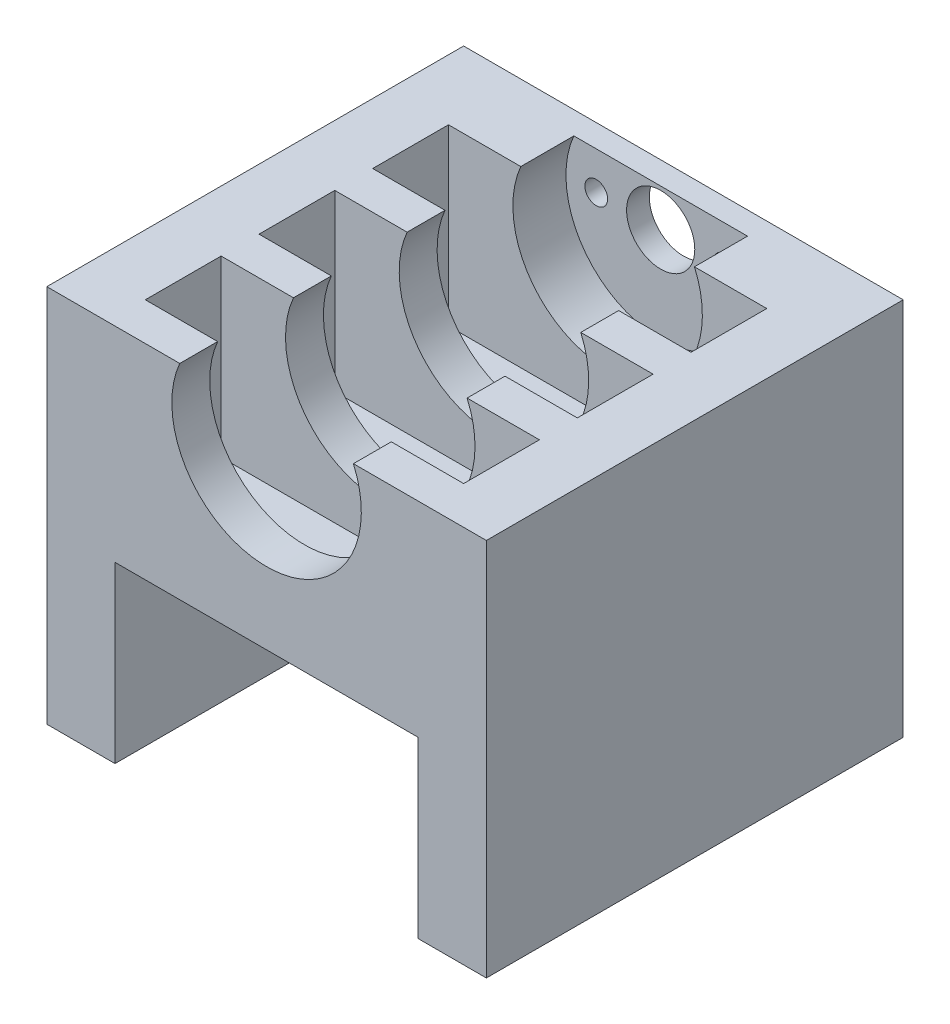
from build123d import *

# Parameters (mm, degrees)
SKETCH1_W             = 58
SKETCH1_H             = 50
BOSS_EXTRUDE1_DEPTH   = 55
SKETCH3_R             = 4.5
SKETCH3_R_2           = 1.5
CUT_EXTRUDE2_DEPTH    = 5
SKETCH2_R             = 12.5
CUT_EXTRUDE1_DEPTH    = 52
SKETCH4_W             = 40
SKETCH4_H             = 46
CUT_EXTRUDE3_DEPTH    = 70
M4_TAPPED_HOLE1_D     = 3.3
M4_TAPPED_HOLE1_DEPTH = 10.1
M4_TAPPED_HOLE1_TIP   = 0.991420021
SKETCH8_W             = 42
SKETCH8_H             = 10
CUT_EXTRUDE4_DEPTH    = 23


with BuildPart() as part:
    # Sketch1 → Boss-Extrude1 (new body)
    with BuildSketch(Plane.XY):
        Rectangle(SKETCH1_W, SKETCH1_H)
    extrude(amount=BOSS_EXTRUDE1_DEPTH)

    # Sketch3 → Cut-Extrude2 (cut)
    with BuildSketch(Plane(origin=(0, 0, 0), x_dir=(-1, 0, 0), z_dir=(0, 0, -1))):
        with Locations((0, 20)):
            Circle(SKETCH3_R)
        with Locations((-8.5, 20)):
            Circle(SKETCH3_R_2)
        with Locations((8.5, 20)):
            Circle(SKETCH3_R_2)
    extrude(amount=-CUT_EXTRUDE2_DEPTH, mode=Mode.SUBTRACT)

    # Sketch2 → Cut-Extrude1 (cut)
    with BuildSketch(Plane.XY.offset(55)):
        with Locations((0, 20)):
            Circle(SKETCH2_R)
    extrude(amount=-CUT_EXTRUDE1_DEPTH, mode=Mode.SUBTRACT)

    # Sketch4 → Cut-Extrude3 (cut)
    with BuildSketch(Plane(origin=(0, 0, 0), x_dir=(-1, 0, 0), z_dir=(0, 0, -1))):
        with Locations((0, -25)):
            Rectangle(SKETCH4_W, SKETCH4_H)
    extrude(amount=-CUT_EXTRUDE3_DEPTH, mode=Mode.SUBTRACT)

    # M4 Tapped Hole1
    with Locations(Plane(origin=(0, -25, 0), x_dir=(-1, 0, 0), z_dir=(0, -1, 0))):
        with Locations((24.5, -47), (24.5, -8), (-24.5, -8), (-24.5, -47)):
            Hole(M4_TAPPED_HOLE1_D / 2, depth=M4_TAPPED_HOLE1_DEPTH)
            with Locations((0, 0, -(M4_TAPPED_HOLE1_DEPTH + M4_TAPPED_HOLE1_TIP / 2))):  # 118° drill point
                Cone(0, M4_TAPPED_HOLE1_D / 2, M4_TAPPED_HOLE1_TIP, mode=Mode.SUBTRACT)

    # Sketch8 → Cut-Extrude4 (cut)
    with BuildSketch(Plane(origin=(0, 25, 0), x_dir=(1, 0, 0), z_dir=(0, 1, 0))):
        with Locations((0, -15)):
            Rectangle(SKETCH8_W, SKETCH8_H)
        with Locations((0, -30)):
            Rectangle(SKETCH8_W, SKETCH8_H)
        with Locations((0, -45)):
            Rectangle(SKETCH8_W, SKETCH8_H)
    extrude(amount=-CUT_EXTRUDE4_DEPTH, mode=Mode.SUBTRACT)


solid = part.part
